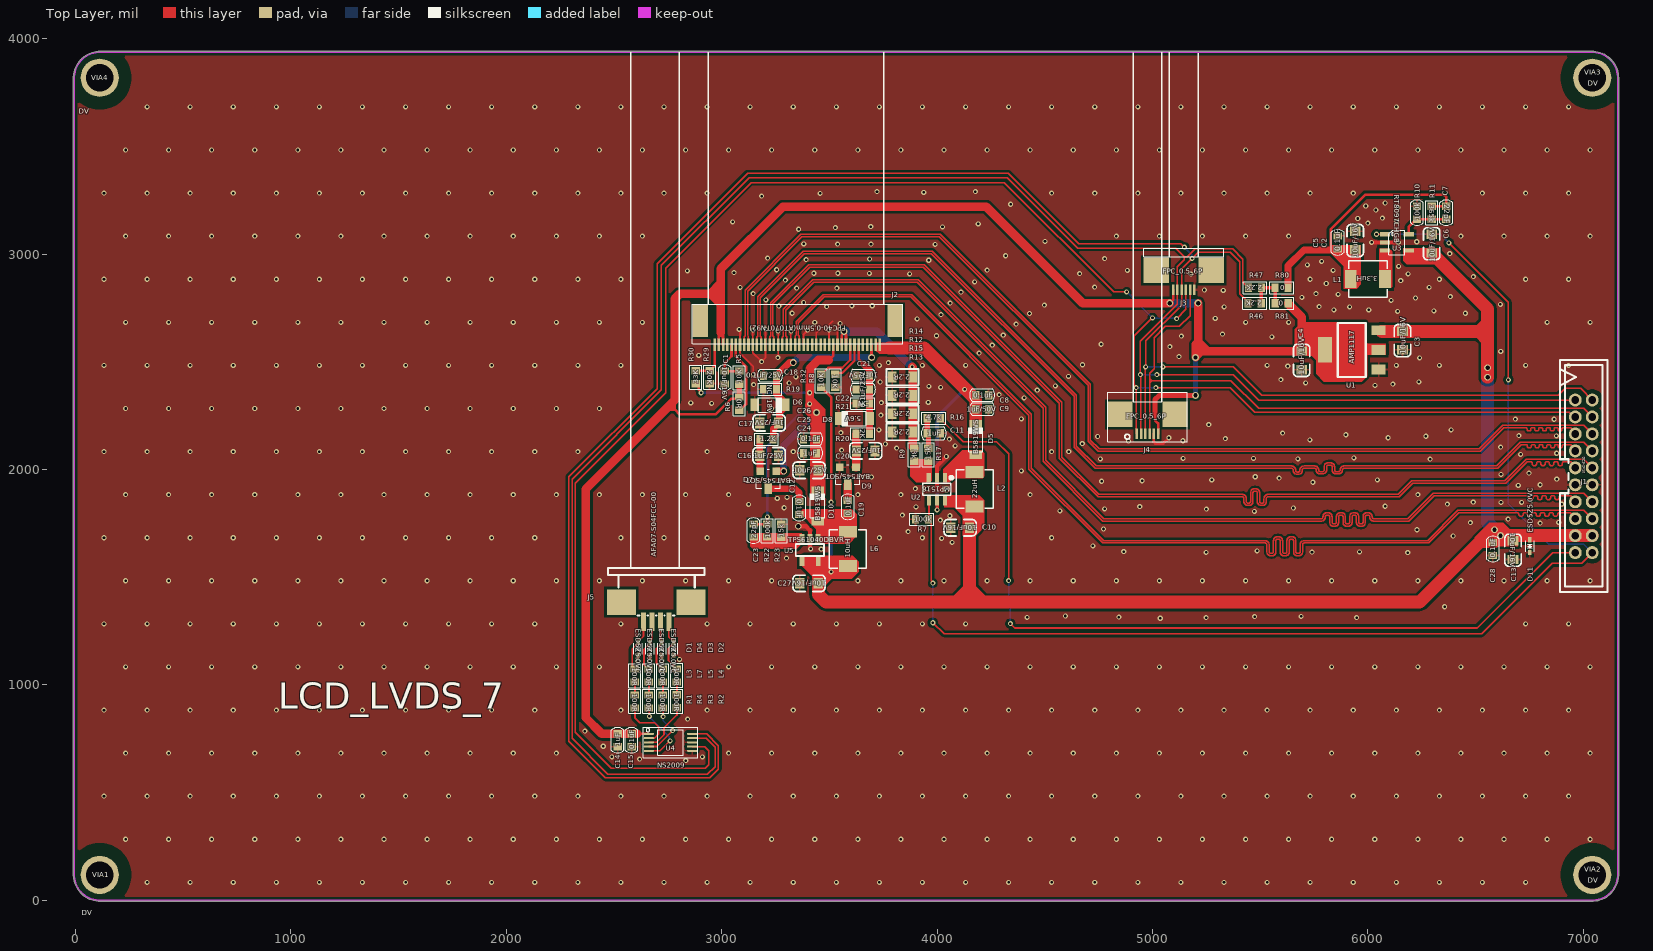
[diagram p0: Top Layer view]
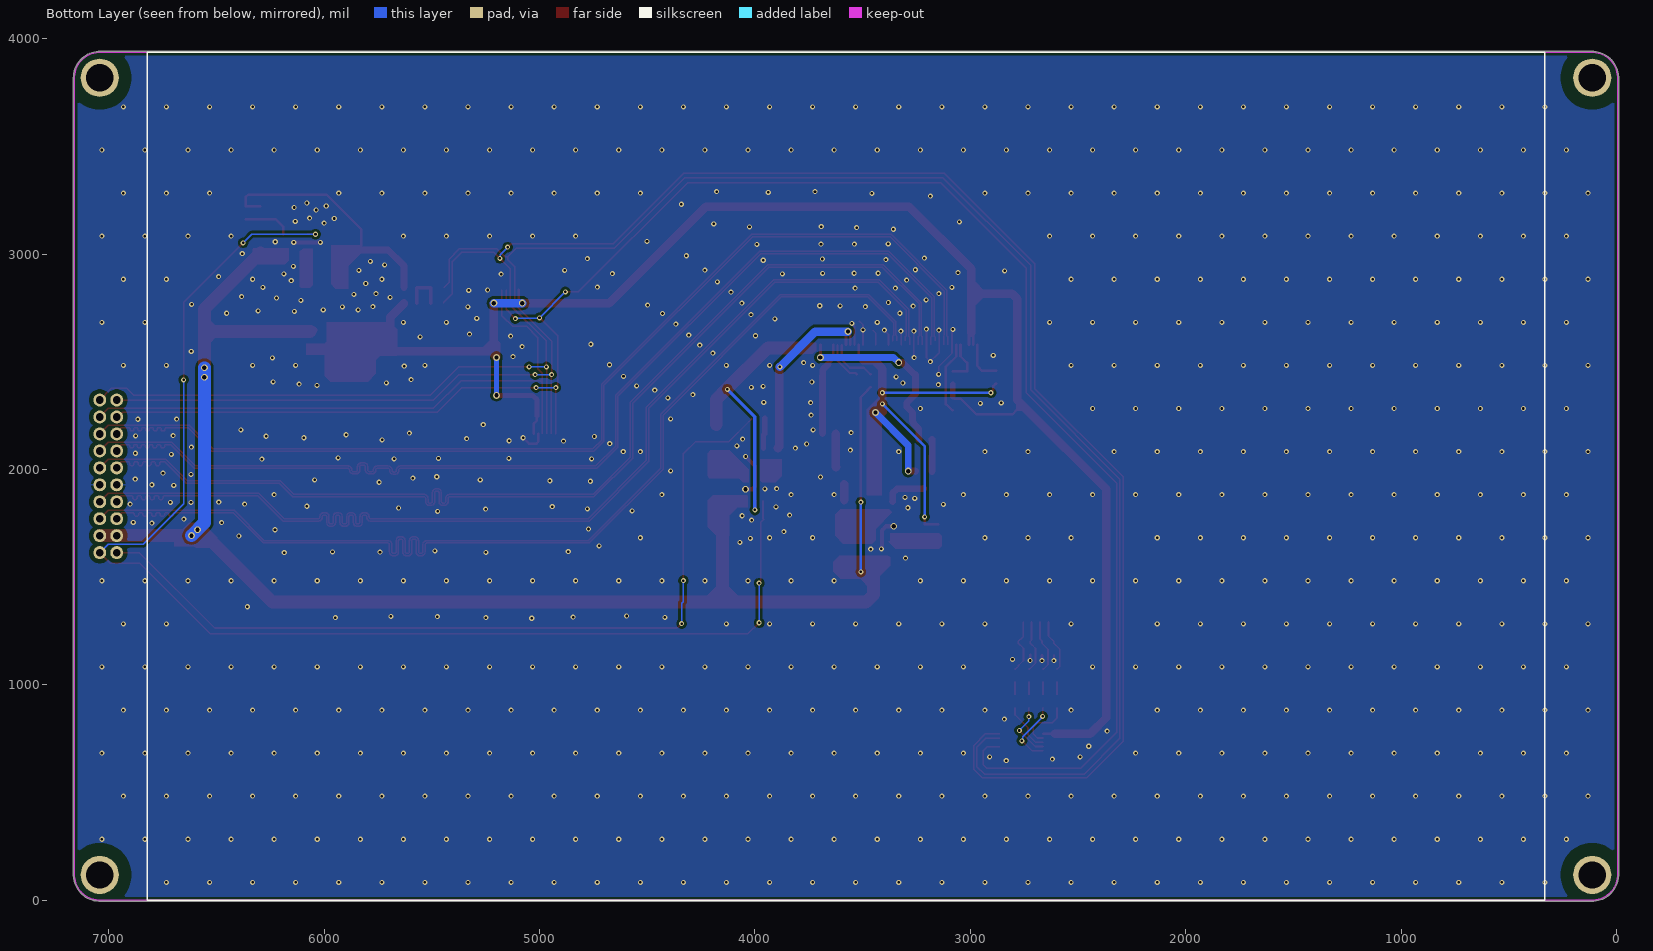
[diagram p1: Bottom Layer view, seen from below]
# Altium PCB MISC82162.PcbDoc (part 1 of 3)
Units mil, origin at the board's own origin, x right, y up, seen from the top; angles counter-clockwise.
Board outline 7173.26 x 3944.91 mil, 2 copper layers (Top Layer, Bottom Layer); 90 components, 54 nets, 272 pads, 794 vias.
Unrouted connection lines stored in the file: 61.

## Layer stack, top to bottom (the 12.6 mil dielectric is the usual default, probably not edited)
Top Solder: solder mask 0.4, Solder Resist, Dk 3.5
Top Layer: signal copper 1.4
Dielectric 1: dielectric 12.6, FR-4, Dk 4.8
Bottom Layer: signal copper 1.4
Bottom Solder: solder mask 0.4, Solder Resist, Dk 3.5

## Board outline
105.73,-4.27 cw(c112.43,117.61) -9.44,110.9 cw(c-5.68,112.09) -9.63,112.09 -9.63,3823.91 cw(c-5.68,3823.91) -9.44,3825.1 cw(c112.43,3818.39) 105.73,3940.27 cw(c106.92,3936.5) 106.92,3940.46 7047.22,3940.46 cw(c7047.22,3936.5) 7048.44,3940.26 cw(c7041.57,3818.39) 7163.63,3818.39 cw(c7041.57,3818.39) 7163.53,3813.49 cw(c7159.68,3812.61) 7163.63,3812.61 7163.63,111.96 cw(c7159.68,111.96) 7163.44,110.74 cw(c7041.57,117.61) 7036.66,-4.36 cw(c7035.79,-0.5) 7035.79,-4.46 106.92,-4.46 cw(c106.92,-0.5)

## Design rules (kind name [scope] priority, off if disabled: settings)
Clearance Clearance_1 [HasFootprint('M3') vs InNet('GND')] p1: gap=5.91 ignorepadtopadclearanceinfootprint=FALSE except(5: Arc-Arc Arc-Track Track-Track; 60: Arc-Fill Arc-Poly Arc-Region Track-Fill Track-Poly Track-Region SMDPad-Fill SMDPad-Poly SMDPad-Region THPad-Fill THPad-Poly THPad-Region Via-Fill Via-Poly Via-Region Fill-Fill Fill-Poly Fill-Region Poly-Poly Poly-Region Region-Region)
Clearance [All] p2: gap=5.91 ignorepadtopadclearanceinfootprint=FALSE except(5: Arc-Arc Arc-Track Track-Track; 11.81: Arc-Fill Arc-Poly Arc-Region Track-Fill Track-Poly Track-Region SMDPad-Fill SMDPad-Poly SMDPad-Region Via-Fill Via-Poly Via-Region Fill-Fill Fill-Poly Fill-Region Poly-Poly Poly-Region Region-Region; 19.68: THPad-Fill THPad-Poly THPad-Region)
DiffPairsRouting [InDifferentialPairClass('LVDS_100R')] p1: maxlimit=5 minlimit=5 mostfreqgap=5 toplayer_minwidth=6 toplayer_maxwidth=6 toplayer_prefwidth=6 bottomlayer_minwidth=6 bottomlayer_maxwidth=6 bottomlayer_prefwidth=6 maxuncoupledlength=500
NetAntennae [All] p1 off: netantennaetolerance=0
PolygonConnect [All] p1: thpad.connectstyle=Relief thpad.reliefconductorwidth=10 thpad.reliefentries=4 thpad.polygonreliefangle="90 Angle" thpad.airgapwidth=10 smdpad.connectstyle=Relief smdpad.reliefconductorwidth=10 smdpad.reliefentries=4 smdpad.polygonreliefangle="90 Angle" smdpad.airgapwidth=10 via.connectstyle=Direct via.reliefconductorwidth=10 via.reliefentries=4 via.polygonreliefangle="90 Angle" via.airgapwidth=10
RoutingVias [All] p1: holewidth=11.81 width=23.62 viastyle="Through Hole" minholewidth=11.81 minwidth=23.62 maxholewidth=19.68 maxwidth=31.5
SilkToSilkClearance [All] p1 off: silktosilkclearance=10
SilkToSolderMaskClearance [IsPad] p1 off: minsilkscreentomaskgap=10 clearancetoexposedcopper=TRUE
SolderMaskExpansion [All] p1: expansion=4 istentingtop=FALSE
Width [All] p1: maxlimit=78.74 minlimit=5.91 preferedwidth=7.87
26 further rules are at their usual default settings.

## Classes and differential pairs
net class LVDS: LVDS0-CLKN LVDS0-CLKP LVDS0-D0N LVDS0-D0P LVDS0-D1N LVDS0-D1P LVDS0-D2N LVDS0-D2P LVDS0-D3N LVDS0-D3P
differential pair class LVDS_100R: D_LVDS0-CLK D_LVDS0-D0 D_LVDS0-D1 D_LVDS0-D2 D_LVDS0-D3
component class POWER: C2 C3 C4 C5 C6 C7 C8 C9 C10 C11 C12 C16 C17 C18 C19 C20 C21 C22 C23 C24 C25 C26 C27 D5 D6 D7 D8 D9 D10 L1 L2 L6 R7 R9 R10 R11 R12 R13 R14 R15 R16 R17 R18 R19 R20 R21 R22 R23 U1 U2 U3 U5 VIA1 VIA2 VIA3 VIA4
component class connect: C1 C13 C14 C15 C28 D1 D2 D3 D4 D11 J1 J2 J3 J4 J5 L3 L4 L5 L7 R1 R2 R3 R4 R5 R6 R8 R29 R30 R32 R46 R47 R80 R81 U4
differential pair D_LVDS0-CLK: +LVDS0-CLKP -LVDS0-CLKN
differential pair D_LVDS0-D0: +LVDS0-D0P -LVDS0-D0N
differential pair D_LVDS0-D1: +LVDS0-D1P -LVDS0-D1N
differential pair D_LVDS0-D2: +LVDS0-D2P -LVDS0-D2N
differential pair D_LVDS0-D3: +LVDS0-D3P -LVDS0-D3N

## Components (designator, comment, footprint, x,y, rotation, side; value= is the part's Value field where it differs from the comment)
C1 "10uF/16V" 0603C 3015,2426.68 r270 top
C2 "10uF/16V" 0805C 5941.25,3062.63 r90 top
C3 "10uF/16V" 0805C 6160.46,2598.23 r270 top
C4 "10uF/16V" 0805C 5692.46,2506.23 r270 top
C5 "0.1uF" 0603C 5859.51,3054.03 r90 top
C6 "10uF/16V" 0805C 6296,3048 r90 top
C7 "22pF" 0603C 6364,3192 r270 top
C8 "0.1uF" 0603C 4209.29,2345.53 r0 top
C9 "1uF/50V" 0603C 4209.29,2280.53 r0 top
C10 "10uF/16V" 0805C 4106.84,1729.43 r180 top
C11 "1uF" 0603C 3984.34,2168.33 r0 top
C12 "0.1uF" 0603C 3360.36,1821.07 r270 top
C13 "10uF/16V" 0805C 6674,1625 r270 top
C14 "1uF" 0603C 2517,743 r270 top
C15 "0.1uF" 0603C 2582,743 r270 top
C16 "1uF/25V" 0805C 3220,2064 r0 top
C17 "1uF/25V" 0805C 3220,2216 r180 top
C18 "0.1uF/25V" 0603C 3224,2436 r180 top
C19 "0.1uF" 0603C 3585.36,1826.07 r90 top
C20 "1uF/25V" 0805C 3668.67,2086.07 r180 top
C21 "1uF/25V" 0603C 3655.36,2436.07 r180 top
C22 "0.1uF/25V" 0603C 3655.36,2371.07 r180 top
C23 "22pF" 0603C 3148,1716 r270 top
C24 "10uF/25V" 0805C 3405.36,1996.07 r180 top
C25 "1uF" 0603C 3410.36,2076.07 r180 top
C26 "0.1uF" 0603C 3410.36,2141.07 r180 top
C27 "10uF/16V" 0805C 3405.36,1471.07 r180 top
C28 "0.1uF" 0603C 6580.43,1630.46 r90 top
D1 "ESD5Z5.0VC" SOD-523 2612,1168 r270 top
D2 "ESD5Z5.0VC" SOD-523 2777,1168 r270 top
D3 "ESD5Z5.0VC" SOD-523 2722,1168 r270 top
D4 "ESD5Z5.0VC" SOD-523 2667,1168 r270 top
D5 "B5819WS" SOD-123 4179.34,2138.33 r90 top
D6 "18V" SOD-123 3224,2300 r0 top
D7 "BAT54S/SOT" SOT23 3216,1952 r180 top
D8 "5.6V" SOD-123 3615.36,2236.07 r180 top
D9 "BAT54S/SOT" SOT23 3585.36,1971.07 r180 top
D10 "B5819WS" SOD-123 3445.36,1831.07 r90 top
D11 "ESD5Z5.0VC" SOD-523 6752,1644 r270 top
J1 "DC3-2*10" DC3-2.0-2*10P 7002.2,1968 r270 top
J2 "FPC40-0.5mm(AT070TN92)" FPC40-0.5MM-UP 3734.48,2558.55 r180 top locked
J3 "FPC_0.5_6P" FPC_0.5_6P_UP 5095.82,2833.94 r0 top locked
J4 "FPC_0.5_6P" FPC_0.5_6P_DOWN 4927.39,2164.85 r0 top locked
J5 "AFA07-S04FCC-00" FPC-SMD-1mm4P-RTP 2695.59,1338.08 r180 top locked
L1 "3.3uH" L-SMD-4*4*1.2 6000,2884 r180 top
L2 "22uH" L-SMD-4*4*1.2 4174.34,1908.33 r90 top
L3 "100R" 0603R 2597,1043 r270 top
L4 "100R" 0603R 2792,1043.51 r270 top
L5 "100R" 0603R 2727,1043 r270 top
L6 "10uH" L-SMD-4*4*1.2 3585.36,1631.07 r90 top
L7 "100R" 0603R 2662,1043 r270 top
R1 "100R" 0603R 2597,923 r270 top
R2 "100R" 0603R 2792,923.51 r270 top
R3 "100R" 0603R 2727,923 r270 top
R4 "100R" 0603R 2662,923 r270 top
R5 "10K" 0603R 3080.72,2426.27 r90 top
R6 "0R" 0603R 3081.7,2305.46 r270 top
R7 "100k" 0603R 3929.34,1768.33 r0 top
R8 "10K" 0603R 3526.99,2411.91 r270 top
R9 "3k" 0603R 3894.34,2068.33 r270 top
R10 "100k" 0603C 6228,3192 r90 top
R11 "365k" 0603R 6296,3192 r270 top
R12 "2.2R" 0805R 3839.34,2343.33 r180 top
R13 "2.2R" 0805R 3839.34,2173.33 r180 top
R14 "2.2R" 0805R 3839.34,2428.33 r180 top
R15 "2.2R" 0805R 3839.34,2258.33 r180 top
R16 "4.7k" 0603R 3984.34,2238.33 r0 top
R17 "15k" 0603R 3959.34,2068.33 r90 top
R18 "1.2K" 0603R 3208,2140 r0 top
R19 "NC" 0603R 3224,2372 r0 top
R20 "2K" 0603R 3655.36,2166.07 r0 top
R21 "NC" 0603R 3655.36,2306.07 r0 top
R22 "100k" 0603R 3212,1716 r90 top
R23 "15k" 0603R 3276.36,1715.07 r270 top
R29 "20K" 0603R 2944,2428 r270 top
R30 "33K" 0603R 2880,2428 r90 top
R32 "10K" 0603R 3461.99,2411.91 r90 top
R46 "2.2K" 0603R 5474.38,2772.16 r180 top
R47 "2.2K" 0603R 5476,2844 r180 top
R80 "0" 0603R 5599.38,2844.16 r0 top
R81 "0" 0603R 5600,2772 r180 top
U1 "AMP1117" SOT223 5925.39,2554.92 r90 top
U2 "MP1518" SOT-23-6 3999.34,1908.33 r180 top
U3 "RT8097CHGB" SOT23-5 6134.51,3054.03 r270 top
U4 "NS2009" MSOP-10 2762,733 r0 top
U5 "TPS61040DBVR" SOT-23-5 3410.36,1626.07 r180 top
VIA1 "DV" M3#1 112,113 r0 top
VIA2 "DV" M3#2 7042,103 r0 top
VIA3 "DV" M3#3 7037,3823 r0 top
VIA4 "DV" M3#4 97,3833 r0 top

## Footprints (in the part's own frame and the unit in brackets; to place one, negate y for a bottom-side part, rotate by r counter-clockwise, add the part's x,y. Pads: shape width x height; smd on the part's side, far side on the other; paste and mask are expansions set on the pad)
0603C [mm]
  rect 0.85x1 smd: 1(-0.77,0) 2(0.77,0)
  silkscreen extent -1.49,-0.76 1.49,0.74
0603R [mm]
  rect 0.85x1 smd: 1(-0.77,0) 2(0.77,0)
  silkscreen extent -1.41,-0.7 1.41,0.7
0805C [mm]
  rect 1.1x1.27 smd: 1(-1.1,0) 2(1.1,0)
  silkscreen extent -1.89,-0.97 1.89,0.97
0805R [mil]
  rect 40x50 smd: 1(-47.28,-0.31) 2(47.21,-0.31)
  silkscreen extent -75,-38 74,38
DC3-2.0-2*10P [mil]
  round 60 hole 36: 1(-354.35,-39.37) 2(-354.35,39.37) 3(-275.55,-39.37) 4(-275.59,39.37) 5(-196.85,-39.37) 6(-196.85,39.37) 7(-118.15,-39.37) 8(-118.11,39.37) 9(-39.35,-39.37) 10(-39.37,39.37) 11(39.35,-39.37) 12(39.37,39.37) 13(118.15,-39.37) 14(118.11,39.37) 15(196.85,-39.37) 16(196.85,39.37) 17(275.55,-39.37) 18(275.59,39.37) 19(354.35,-39.37) 20(354.33,39.37)
  silkscreen extent -540,-110 537,110
FPC40-0.5MM-UP [mm]
  rect 0.3x1.5 smd: 1(19.5,-0.5) 2(19,-0.5) 3(18.5,-0.5) 4(18,-0.5) 5(17.5,-0.5) 6(17,-0.5) 7(16.5,-0.5) 8(16,-0.5) 9(15.5,-0.5) 10(15,-0.5) 11(14.5,-0.5) 12(14,-0.5) 13(13.5,-0.5) 14(13,-0.5) 15(12.5,-0.5) 16(12,-0.5) 17(11.5,-0.5) 18(11,-0.5) 19(10.5,-0.5) 20(10,-0.5) 21(9.5,-0.5) 22(9,-0.5) 23(8.5,-0.5) 24(8,-0.5) 25(7.5,-0.5) 26(7,-0.5) 27(6.5,-0.5) 28(6,-0.5) 29(5.5,-0.5) 30(5,-0.5) 31(4.5,-0.5) 32(4,-0.5) 33(3.5,-0.5) 34(3,-0.5) 35(2.5,-0.5) 36(2,-0.5) 37(1.5,-0.5) 38(1,-0.5) 39(0.5,-0.5) 40(0,-0.5)
  rect 1.8x3.8 smd: 41(-1.796,-3.345) 42(21.191,-3.35)
  silkscreen extent -2.71,-5.28 22.1,-0.63
FPC-SMD-1mm4P-RTP [mm]
  rect 0.6x2.2 smd: 1(1.499,1.163) 2(0.499,1.163) 3(-0.5,1.163) 4(-1.5,1.163)
  rect 3.4x3 smd: 5(-4.1,-1.162) 6(4.1,-1.163)
  silkscreen extent -5.72,-5.19 5.69,0.42
FPC_0.5_6P_DOWN [mm]
  rect 0.3x1.25 smd: 1(0,0) 2(0.5,0) 3(1,0) 4(1.5,0) 5(2,0) 6(2.5,0)
  rrect0% 3x3 smd: 7(-2,2.3) 8(4.5,2.3)
  silkscreen extent -3.44,-0.93 5.93,4.9
FPC_0.5_6P_UP [mm]
  rect 0.3x1.25 smd: 1(0,0) 2(0.5,0) 3(1,0) 4(1.5,0) 5(2,0) 6(2.5,0)
  rrect0% 3x3 smd: 7(-2,2.3) 8(4.5,2.3)
  silkscreen extent -3.44,3.9 5.99,4.9
L-SMD-4*4*1.2 [mm]
  rect 1.4x2.12 smd: 1(-2.028,0) 2(2.028,0)
  silkscreen extent -2.28,-2.18 2.28,2.18
M3#1 [mm]
  round 4.5 hole 3.2: 1(0.011,0.117)
M3#2 [mm]
  round 4.5 hole 3.2: 1(-0.011,0.371)
M3#3 [mm]
  round 4.5 hole 3.2: 1(0.116,-0.117)
M3#4 [mm]
  round 4.5 hole 3.2: 1(0.392,-0.371)
MSOP-10 [mm]
  oval 1.2x0.25 smd paste-0.1 mask-0.1: 1(-2.55,1) 2(-2.55,0.5) 3(-2.55,0) 4(-2.55,-0.5) 5(-2.55,-1) 6(2.55,-1) 7(2.55,-0.5) 8(2.55,0) 9(2.55,0.5) 10(2.55,1)
  silkscreen extent -3.2,-1.8 3.2,1.8
SOD-123 [mm]
  rect 1x1.5 smd: 1(-1.8,0) 2(1.8,0)
  silkscreen extent -1.4,-0.85 1.4,0.85
SOD-523 [mm]
  rect 0.6x0.4 smd: 1(-0.75,0) 2(0.75,0)
  silkscreen extent -0.65,-0.5 0.65,0.5
SOT23 [mil]
  rect 36x36 smd: 1(-37.5,-39) 2(37.5,-39)
  rect 36x50 smd: 3(0,41)
  silkscreen extent -55,-50 55,40
SOT23-5 [mm]
  rect 0.5x1.2 smd: 1(-0.95,-1.4) 2(0,-1.4) 3(0.95,-1.4) 4(0.95,1.4) 5(-0.95,1.4)
  silkscreen extent -1.45,-0.95 1.45,0.95
SOT223 [mil]
  rect 45x65 smd: 1(-91,-125) 2(0,-125) 3(91,-125)
  rect 118x65 smd: 4(0,125)
  silkscreen extent -125,-65 125,65
SOT-23-5 [mm]
  rect 0.6x1.1 smd: 1(-0.951,-1.347) 2(0.009,-1.347) 3(0.969,-1.347)
  rect 0.55x1.1 smd: 4(0.954,1.353) 5(-0.951,1.353)
  silkscreen extent -1.63,-0.7 1.69,0.71
SOT-23-6 [mm]
  rect 0.5x1.1 smd: 1(-0.96,-1.35) 2(0,-1.35) 3(0.96,-1.35) 4(0.945,1.35) 5(0,1.35) 6(-0.96,1.35)
  silkscreen extent -1.79,-1.45 1.68,0.71

## Part data
C1 C3 C4 C10 C12 C18 C19 C21 C22: library part C
C2: library part CAPACITOR_0
C5 C6 C7: library part CAPACITOR
C8 C11 C14 C15 C23 C25 C26 C28: library part CAP, "Capacitor"
C9: library part C_Dup1
C13 C16 C17 C20 C24 C27: library part "CAP POL"
D1 D2 D3 D4 D11: library part 1_1.5KE100A
D5 D10: library part BAS21/SOT_1
D6 D8: library part "DIODE BREAKDOWN_1"
J2: library part "HEADER 20X2_3"
J3 J4: library part connet_0
J5: library part AFC07-S04ECC-00, JLCPCB Part Class="Extended Part", LCSC Part Name="0.5mm P数:4 抽屉式 上接", Manufacturer=JS(钜硕电子)
L1: library part "INDUCTOR IRON"
L2 L3 L4 L5 L7: library part INDUCTOR
L6: library part "CHOKE TORROID-FERRITE"
R1 R2 R3 R4 R7 R9 R12 R13 R14 R15 R16 R17 R22 R23: library part RES2
R5 R6 R8 R10 R11 R29 R30 R32 R46 R47 R80 R81: library part R
R18 R19 R20 R21: library part RESISTOR
U1: library part LM7805/TO_6
U2: library part PT4110_0
U3: library part XC9235_0
U5: library part X9C102/SO_2
VIA1 VIA2 VIA3 VIA4: library part DV_0

## Via types
v1: diameter 23.62, hole 11.81, Top Layer to Bottom Layer, 779 vias
v2: diameter 32, hole 20, Top Layer to Bottom Layer, 13 vias
v3: diameter 31.5, hole 19.68, Top Layer to Bottom Layer, 2 vias

## Nets (pads, with @x,y where several pads share a name; then routed paths per layer and width w, separated by ;. In a path a pad name is that pad's centre, name@x,y a point inside that pad or via, vN(x,y) a via of type N, cw(c..) or ccw(c..) an arc to the next point about the centre after c; other vN are vias at no path point)
AVDD: C23.1 C24.1 C25.1 C26.1 D7.1 D10.2 J2.29 R22.2 R30.1 | length 2398.3
  Top Layer w12: R30.1@2880,2397.68 2882.95,2397.68 2893.69,2386.95 2893.69,2369.46 2904,2359.14 v1(2904,2356) ; C23.1@3148,1746.32 R22.2@3212,1746.32 v1(3212,1780) ; 3496,2508 3517.94,2529.94 J2.29@3517.94,2578.24
  Top Layer w32: D7.1@3253.5,1991 3254.5,1992 v2(3288,1992) ; 3440.68,2226.7 C26.1@3440.68,2141.07 C25.1@3440.68,2076.07 3440.68,2073.12 3448.67,2065.13 C24.1@3448.67,1996.07 3447.02,1994.42 3447.02,1903.59 D10.2@3445.36,1901.94
  Top Layer w40: 3440.68,2226.7 3440.68,2247.32 3408,2280 v1(3408,2304) v1(3408,2356) 3408,2468 3448,2508 3496,2508
  Bottom Layer w12: v1(2904,2356) v1(3408,2356) ; v1(3212,1780) 3212,2108 v1(3408,2304)
  Bottom Layer w32: v2(3288,1992) 3288,2112 v2(3440,2264)
AVDD2.8V: C2.1 C5.1 C7.1 L1.2 R11.1 R80.2 | length 1284.2
  Top Layer w12: C5.1@5859.51,3023.71 5828.29,3023.71 5827.91,3024.09 5827.91,3115.91 5988,3276 6352,3276 6364,3264 C7.1@6364,3222.31 R11.1@6296,3222.31
  Top Layer w32: R80.2@5629.7,2844.16 5629.7,2945.7 5703.32,3019.32 5828.29,3019.32 5856.55,3019.32 C2.1@5941.25,3019.32
CTP_INT: J1.3 J3.4 J4.1 U4.7 | length 8801.7
  Top Layer w6: U4.7@2862.39,713.32 2920.68,713.32 2940,694 2940,628 2924,612 2488,612 2320,780 2320,1936 2739.06,2355.06 2739.06,2935.06 3136,3332 4312,3332 4820,2824 v1(4880,2824) ; J4.1@4927.39,2164.85 4925.7,2166.55 4925.7,2382.63 4916,2392.33 4916,2620.61 4999.39,2704 v1(5000,2704) ; v1(5016,2380) 5360,2380 5475,2265 6934.09,2265 6955.54,2243.55 J1.3@6962.83,2243.55 ; v1(5112,2700) 5154.87,2742.87 J3.4@5154.87,2833.94
  Bottom Layer w6: v1(4880,2824) v1(5000,2704) 5002,2702 5110,2702 v1(5112,2700) ; v1(4924,2380) v1(5016,2380)
CTP_RST: J1.4 J3.5 J4.4 | length 2944.1
  Top Layer w6: J4.4@4986.45,2164.85 4986.45,2402.45 ; 4986.45,2429.22 4986.45,2421.55 ; J3.5@5174.56,2833.94 5174.56,2714.56 5124,2664 5060,2664 5008,2612 5008,2468 4986.45,2446.45 4986.45,2421.55 ; J1.4@7041.57,2243.59 7001.71,2283.44 5492.56,2283.44 5364,2412 4996,2412 ; 4986.45,2402.45 4986.45,2412 ; 4986.45,2402.45 4996,2412 ; 4986.45,2412 4996,2412 ; 4986.45,2412 4986.45,2421.55 ; 4986.45,2421.55 4996,2412
CTP_TWI1_SCK: J1.2 J3.3 J4.3 R46.2 U4.10 | length 9781.4
  Top Layer w6: U4.10@2862.39,772.37 2930.63,772.37 2985,718 2985,609 2944,568 2460,568 2290,738 2290,1965 2700,2375 2700,2955 3120,3375 4330,3375 4657,3048 5132,3048 v1(5148,3032) ; J4.3@4966.76,2164.85 4966.76,2474.76 v1(4968,2476) 4968.72,2476.72 4968.72,2596.72 5135.19,2763.19 J3.3@5135.19,2833.94 5135.19,2931.19 v1(5184,2980) 5212,3008 5360,3008 5404,2964 5404,2815.18 5444.07,2775.11 R46.2@5444.07,2772.16 ; v1(5048,2476) 5376,2476 5508,2344 6884,2344 6916,2376 6987.92,2376 J1.2@7041.57,2322.35
  Bottom Layer w6: v1(4968,2476) v1(5048,2476) ; v1(5148,3032) 5183.28,2996.72 5183.28,2980.72 v1(5184,2980)
CTP_TWI1_SDA: J1.1 J3.2 J4.2 R47.2 U4.9 | length 9506.5
  Top Layer w6: U4.9@2862.39,752.68 2927.32,752.68 2969,711 2969,620.56 2932.6,584.16 2471.68,584.16 2305,750.84 2305,1955 2719.69,2369.69 2719.69,2946.85 3128.15,3355.31 4324.69,3355.31 4652,3028 5107.5,3028 5147.75,2987.75 ; J4.2@4947.08,2164.85 4945.54,2166.39 4945.54,2438.46 v1(4944,2440) 4944,2596 5115.5,2767.5 J3.2@5115.5,2833.94 5115.5,2940.8 5147.75,2973.05 5147.75,2987.75 ; v1(5020,2440) 5376,2440 5493.65,2322.35 J1.1@6962.83,2322.35 ; R47.2@5445.69,2844 5420,2869.68 5420,2976 5372,3024 5198.7,3024 5161.35,2986.65 5148.86,2986.65 5147.75,2987.75
  Bottom Layer w6: v1(4944,2440) v1(5020,2440)